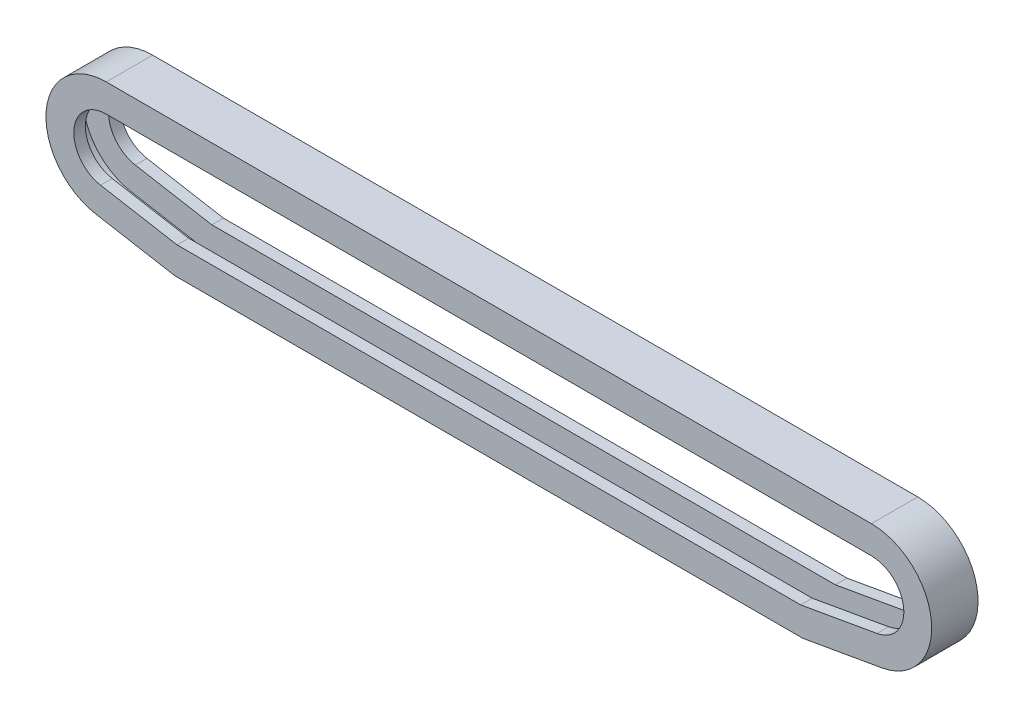
from build123d import *

# Parameters (mm, degrees)
BOSS_EXTRUDE1_DEPTH = 10
CUT_EXTRUDE1_DEPTH  = 5


with BuildPart() as part:
    # Sketch2 → Boss-Extrude1 (new, symmetric)
    with BuildSketch(Plane.XY):
        with BuildLine():
            Line((-165, 26), (165, 26))
            ThreePointArc((165, 26), (190.90106215, 2.266049311), (169.514852619, -25.605001578))
            Line((169.514852619, -25.605001578), (135.524931981, -31.598341659))
            Line((135.524931981, -31.598341659), (-135.524931981, -31.598341659))
            Line((-135.524931981, -31.598341659), (-169.514852619, -25.605001578))
            ThreePointArc((-169.514852619, -25.605001578), (-190.90106215, 2.266049311), (-165, 26))
        make_face()
        with BuildLine():
            Line((-165, 14), (165, 14))
            ThreePointArc((165, 14), (178.946725773, 1.220180398), (167.431074487, -13.787308542))
            Line((167.431074487, -13.787308542), (134.475068019, -19.598341659))
            Line((134.475068019, -19.598341659), (-134.475068019, -19.598341659))
            Line((-134.475068019, -19.598341659), (-167.431074487, -13.787308542))
            ThreePointArc((-167.431074487, -13.787308542), (-178.946725773, 1.220180398), (-165, 14))
        make_face(mode=Mode.SUBTRACT)
    extrude(amount=BOSS_EXTRUDE1_DEPTH, both=True)

    # Sketch8 → Cut-Extrude1 (cut, symmetric)
    with BuildSketch(Plane.XY):
        with BuildLine():
            Line((135.437443318, -30.598341659), (169.341204442, -24.620193825))
            ThreePointArc((169.341204442, -24.620193825), (189.904867452, 2.178893569), (165, 25))
            Line((165, 25), (-165, 25))
            ThreePointArc((-165, 25), (-189.904867452, 2.178893569), (-169.341204442, -24.620193825))
            Line((-169.341204442, -24.620193825), (-135.437443318, -30.598341659))
            Line((-135.437443318, -30.598341659), (135.437443318, -30.598341659))
        make_face()
    extrude(amount=CUT_EXTRUDE1_DEPTH, both=True, mode=Mode.SUBTRACT)


solid = part.part
